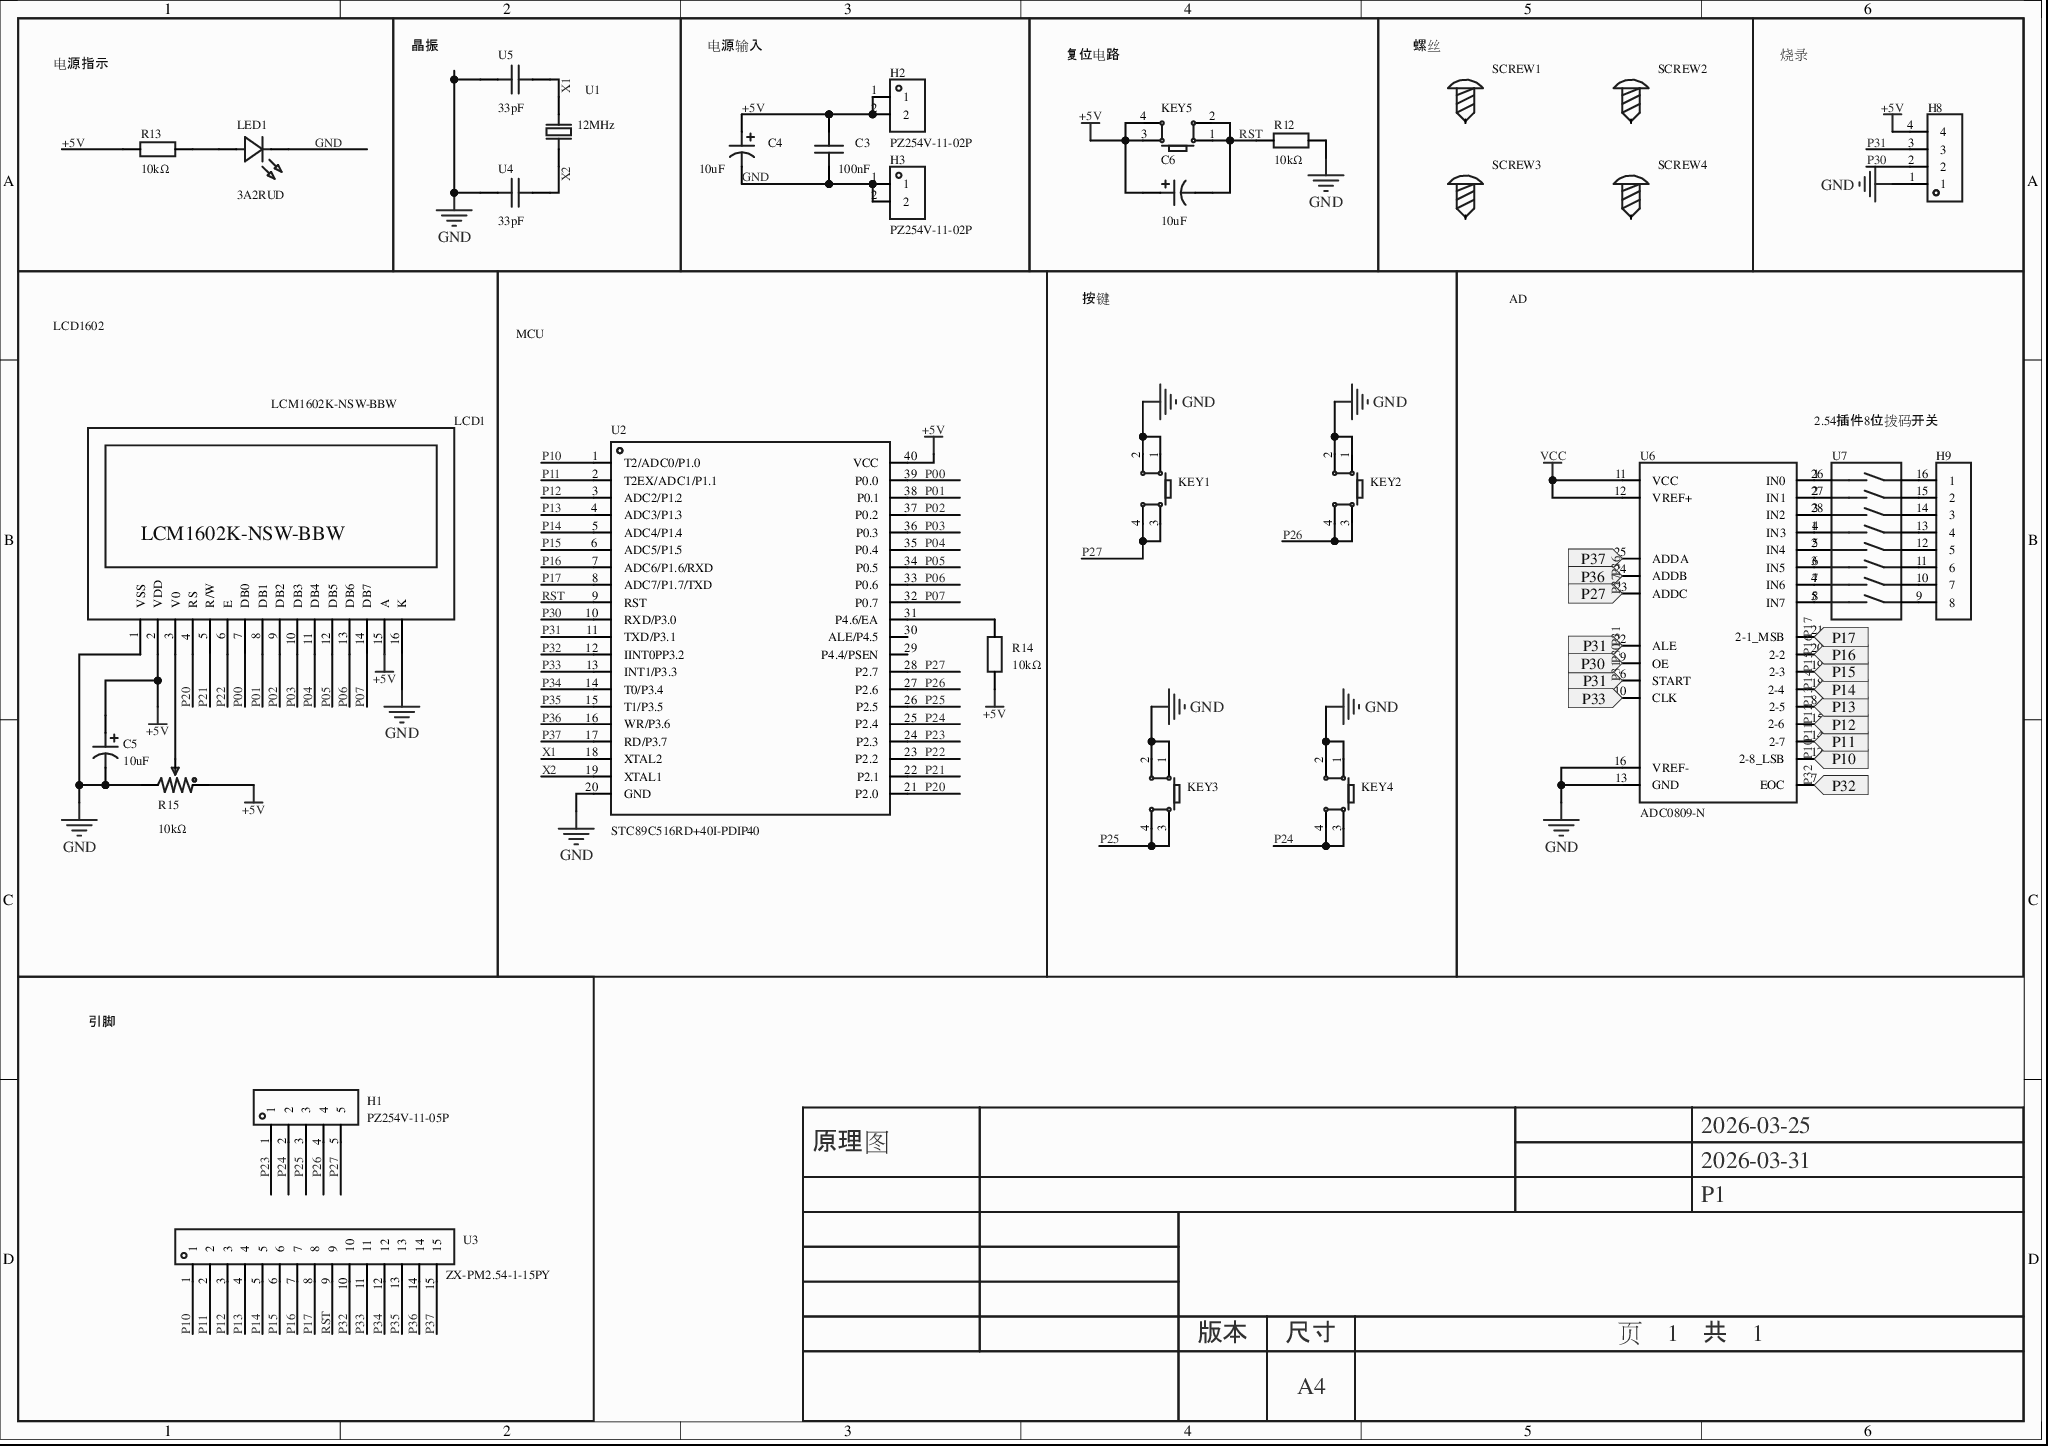
[diagram p0: MISC51962-3.schdoc]
# Altium project MISC51962-2.PrjPcb
1 sheet, 31 parts. Net scope: flat (ports and power ports of the same name join across sheets).
Board file: MISC51962.pcbdoc

## Sheet MISC51962-3.schdoc
size 297 x 209 mm; Version: V1.0; @Project Name: MISC51962; @Page Count: 1; @Update Date: 2026-04-15; @Create Date: 2026-04-15; @Schematic Name: MISC51962; @Page No: 1; @Board Name: MISC51962; @Create Time: 20:25:54; @Update Time: 20:28:01; Size: A4

### Parts
C3  100nF  [CAP-TH_L5.0-W2.5-P5.00-D1.0]
C4  10uF  [CAP-TH_BD5.0-P2.00-D0.5-FD-A]
C5  10uF  [CAP-TH_BD5.0-P2.00-D0.5-FD-A]
C6  10uF  [CAP-TH_BD5.0-P2.00-D0.5-FD-A]
H1  PZ254V-11-05P  [HDR-TH_5P-P2.54-V-M]
H2  PZ254V-11-02P  [HDR-TH_2P-P2.54-V-M]
H3  PZ254V-11-02P  [HDR-TH_2P-P2.54-V-M]
H8  (no value)  [HDR-TH_4P-P2.54-V-F]
H9  (no value)  [HDR-TH_8P-P2.54-V-F-1]
KEY1  (no value)  [SW-TH_4P-L6.0-W6.0-P4.50-LS6.5]
KEY2  (no value)  [SW-TH_4P-L6.0-W6.0-P4.50-LS6.5]
KEY3  (no value)  [SW-TH_4P-L6.0-W6.0-P4.50-LS6.5]
KEY4  (no value)  [SW-TH_4P-L6.0-W6.0-P4.50-LS6.5]
KEY5  (no value)  [SW-TH_4P-L6.0-W6.0-P4.50-LS6.5]
LCD1  LCM1602K-NSW-BBW  [MODULE-TH_LCM1602K]
LED1  3A2RUD  [LED-TH_BD3.5-P2.28_3A2RUC]
R12  10kΩ  [RES-TH_BD2.3-L6.5-P10.50-D0.5]
R13  10kΩ  [RES-TH_BD2.3-L6.5-P10.50-D0.5]
R14  10kΩ  [RES-TH_BD2.3-L6.5-P10.50-D0.5]
R15  10kΩ  [RES-ADJ-TH_3P-L10.0-W10.0-P2.50-L]
SCREW1  (no value)  [M3螺丝]
SCREW2  (no value)  [M3螺丝]
SCREW3  (no value)  [M3螺丝]
SCREW4  (no value)  [M3螺丝]
U1  12MHz  [HC-49S_L11.0-W4.7-P4.88]
U2  STC89C516RD+40I-PDIP40  [DIP-40_L52.3-W13.9-P2.54-LS15.2-BL]
U3  ZX-PM2.54-1-15PY  [HDR-TH_15P-P2.54-V-F]
U4  33pF  [CAP-TH_L5.0-W2.5-P5.08-D0.7]
U5  33pF  [CAP-TH_L5.0-W2.5-P5.08-D0.7]
U6  ADC0809-N  [PDIP-28_L36.0-W13.0-P2.54-LS15.5-BL]
U7  2.54插件8位拨码开关  [SW-TH_16P-L21.9-W9.9-P2.54-LS7.8]

### Blocks framed on the sheet
电源指示: LED1 R13
晶振: U1 U4 U5
电源输入: C3 C4 H2 H3
复位电路: C6 KEY5 R12
螺丝: SCREW1-SCREW4
烧录: H8
LCD1602: C5 LCD1 R15
MCU: R14 U2
按键: KEY1-KEY4
AD: H9 U6 U7
引脚: H1 U3

### Ports
P10 (in), P11 (in), P12 (in), P13 (in), P14 (in), P15 (in), P16 (in), P17 (in), P27 (in), P30 (in), P31 (in), P32 (in), P33 (in), P36 (in), P37 (in)

### Nets
+5V: C3.2 C4.1 C5.1 C6.1 H2.1 H2.2 H8.4 KEY5.3 KEY5.4 LCD1.2(VDD) LCD1.15(A) R13.2 R14.1 R15.1 U2.40(VCC)
GND: C3.1 C4.2 C5.2 H3.1 H3.2 H8.1 KEY1.1 KEY1.2 KEY2.1 KEY2.2 KEY3.1 KEY3.2 KEY4.1 KEY4.2 LCD1.1(VSS) LCD1.16(K) LED1.1(K) R12.1 R15.3 U2.20(GND) U4.1 U5.1 U6.13(GND) U6.16(VREF-)
VCC: U6.11(VCC) U6.12(VREF+)
P00: LCD1.7(DB0) U2.39(P0.0)
P01: LCD1.8(DB1) U2.38(P0.1)
P02: LCD1.9(DB2) U2.37(P0.2)
P03: LCD1.10(DB3) U2.36(P0.3)
P04: LCD1.11(DB4) U2.35(P0.4)
P05: LCD1.12(DB5) U2.34(P0.5)
P06: LCD1.13(DB6) U2.33(P0.6)
P07: LCD1.14(DB7) U2.32(P0.7)
P10: U2.1(T2/ADC0/P1.0) U3.1 U6.17(2-8_LSB) ; port P10
P11: U2.2(T2EX/ADC1/P1.1) U3.2 U6.14(2-7) ; port P11
P12: U2.3(ADC2/P1.2) U3.3 U6.15(2-6) ; port P12
P13: U2.4(ADC3/P1.3) U3.4 U6.8(2-5) ; port P13
P14: U2.5(ADC4/P1.4) U3.5 U6.18(2-4) ; port P14
P15: U2.6(ADC5/P1.5) U3.6 U6.19(2-3) ; port P15
P16: U2.7(ADC6/P1.6/RXD) U3.7 U6.20(2-2) ; port P16
P17: U2.8(ADC7/P1.7/TXD) U3.8 U6.21(2-1_MSB) ; port P17
P20: LCD1.4(RS) U2.21(P2.0)
P21: LCD1.5(R/W) U2.22(P2.1)
P22: LCD1.6(E) U2.23(P2.2)
P23: H1.1 U2.24(P2.3)
P24: H1.2 KEY4.3 KEY4.4 U2.25(P2.4)
P25: H1.3 KEY3.3 KEY3.4 U2.26(P2.5)
P26: H1.4 KEY2.3 KEY2.4 U2.27(P2.6)
P27: H1.5 KEY1.3 KEY1.4 U2.28(P2.7) U6.23(ADDC) ; port P27
P30: H8.2 U2.10(RXD/P3.0) U6.9(OE) ; port P30
P31: H8.3 U2.11(TXD/P3.1) U6.6(START) U6.22(ALE) ; port P31
P32: U2.12(IINT0PP3.2) U3.10 U6.7(EOC) ; port P32
P33: U2.13(INT1/P3.3) U3.11
P34: U2.14(T0/P3.4) U3.12
P35: U2.15(T1/P3.5) U3.13
P36: U2.16(WR/P3.6) U3.14 U6.24(ADDB) ; port P36
P37: U2.17(RD/P3.7) U3.15
RST: C6.2 KEY5.1 KEY5.2 R12.2 U2.9(RST) U3.9
X1: U1.2 U2.18(XTAL2) U5.2
X2: U1.1 U2.19(XTAL1) U4.2
NetH9_1: H9.1 U7.16
NetH9_2: H9.2 U7.15
NetH9_3: H9.3 U7.14
NetH9_4: H9.4 U7.13
NetH9_5: H9.5 U7.12
NetH9_6: H9.6 U7.11
NetH9_7: H9.7 U7.10
NetH9_8: H9.8 U7.9
NetLCD1_3: LCD1.3(V0) R15.2
NetLED1_2: LED1.2(A) R13.1
NetR14_2: R14.2 U2.31(P4.6/EA)
NetU6_1: U6.1(IN3) U7.4
NetU6_2: U6.2(IN4) U7.5
NetU6_3: U6.3(IN5) U7.6
NetU6_4: U6.4(IN6) U7.7
NetU6_5: U6.5(IN7) U7.8
NetU6_10: U6.10(CLK) ; port P33
NetU6_25: U6.25(ADDA) ; port P37
NetU6_26: U6.26(IN0) U7.1
NetU6_27: U6.27(IN1) U7.2
NetU6_28: U6.28(IN2) U7.3

Not connected (* = marked no-connect by the designer): SCREW1 1*; SCREW2 1*; SCREW3 1*; SCREW4 1*; U2 29(P4.4/PSEN)* 30(ALE/P4.5)*

### Notes on the sheet
- 2026-03-25
- 原理图
- 2026-03-31
- P1
- 版本
- 尺寸
- A4
- 页    1    共    1

### Library data of the parts
C3 = CC1H104MC1FD3F6C10MF: Manufacturer: Dersonic(德尔创); AddInBom: yes; Tolerance: ±20%; Voltage Rating: 50V; Pin Spacing: 5.08mm; Temperature Coefficient: Y5V; Body Thickness: 2.2mm; ModelId: 08e3d7481fc7486bb1b263873f51e1e1; ModelName: CAP-TH_BD5.0-W2.5-P5.08; ModelTransform: 224.652,98.425,0,0,0,0,-0.005,0,-137.795; Device: CC1H104MC1FD3F6C10MF; Symbol: CC1H104MC1FD3F6C10MF; FootprintName: CAP-TH_L5.0-W2.5-P5.00-D1.0; LCSC Part Name: 100nF ±20% 50V; SupplierPart: C254085; ManufacturerPart: CC1H104MC1FD3F6C10MF; Supplier Footprint: 插件,P=5.08mm; JLCPCB Part Class: 扩展库; Datasheet: https://item.szlcsc.com/datasheet/CC1H104MC1FD3F6C10MF/248635.html; Supplier: LCSC; ConvertToPcb: yes; Value: 100nF; Diameter: 6mm
C4-C6 = ERG50V10M5X11: Manufacturer: JIERR(捷而瑞); AddInBom: yes; Tolerance: ±20%; Voltage Rating: 50V; Ripple Current: 180mA@100kHz; Equivalent Series Resistance(ESR): 1.3Ω@100kHz; Pin Spacing: 2mm; Lifetime: 2000hrs@105℃; ModelId: fb608287dcd66704; ModelTransform: 0,0,0,0,0,0,0,0,0; Device: ERG50V10M5X11; Symbol: ERG50V10M5X11; FootprintName: CAP-TH_BD5.0-P2.00-D0.5-FD-A; LCSC Part Name: 10uF ±20% 50V; SupplierPart: C47344184; ManufacturerPart: ERG50V10M5X11; Supplier Footprint: 插件,D5xL11mm; JLCPCB Part Class: 扩展库; Datasheet: https://item.szlcsc.com/datasheet/ERG50V10M5X11/49556625.html; Supplier: LCSC; ConvertToPcb: yes; Value: 10uF; Diameter: 5mm; Height - Seated (Max): 11mm; Operating Temperature: -40℃~+105℃; ModelName: CAP-TH_BD5.0-P2.00-D0.5-FD-A
H1 = PZ254V-11-05P: Manufacturer: XFCN(兴飞); AddInBom: yes; Pin Structure: 1x5P; Pitch: 2.54mm; Circluar Pins/Square Pins: 方针; Current Rating: 3A; Voltage Rating (Max): 250V; ModelId: 47d466e4a34f4fc5bc626cf773a24dd5; ModelName: HDR-TH_5P-P2.54-M-LI-1X5P; ModelTransform: 499.999,100,0,0,0,0,0,0,-118.11; Device: PZ254V-11-05P; Symbol: PZ254V-11-05P; FootprintName: HDR-TH_5P-P2.54-V-M; LCSC Part Name: 1x5P 间距:2.54mm 方针 直插; SupplierPart: C492404; ManufacturerPart: PZ254V-11-05P; Supplier Footprint: 插件,P=2.54mm; JLCPCB Part Class: 扩展库; Datasheet: https://item.szlcsc.com/datasheet/PZ254V-11-05P/502960.html; Supplier: LCSC; ConvertToPcb: yes; Row Spacing: -; Mounting Type: 直插; Number of Rows: 单排; Number of Pins: 5P; Length of Mating Pin: 6mm; Insulation Height: 2.5mm; Length of End Connection Pin: 3mm; Contact Material: 黄铜; Contact Plating: -; Operating Temperature: -40℃~+105℃; Color: 黑色
H2 H3 = PZ254V-11-02P: Manufacturer: XFCN(兴飞); AddInBom: yes; Pin Structure: 1x2P; Pitch: 2.54mm; Circluar Pins/Square Pins: 方针; Current Rating: 3A; Voltage Rating (Max): 250V; ModelId: e35305ec3aa84b66b849f914b715e73f; ModelName: HDR2.54-M-LI-1X2P; ModelTransform: 200,100,0,0,0,0,0,0,-118.11; Device: PZ254V-11-02P; Symbol: PZ254V-11-02P; FootprintName: HDR-TH_2P-P2.54-V-M; LCSC Part Name: 1x2P 间距:2.54mm 方针 直插; SupplierPart: C492401; ManufacturerPart: PZ254V-11-02P; Supplier Footprint: 插件,P=2.54mm; JLCPCB Part Class: 扩展库; Datasheet: https://item.szlcsc.com/datasheet/PZ254V-11-02P/502957.html; Supplier: LCSC; ConvertToPcb: yes; Row Spacing: -; Mounting Type: 直插; Number of Rows: 单排; Number of Pins: 2P; Length of Mating Pin: 6mm; Insulation Height: 2.5mm; Length of End Connection Pin: 3mm; Contact Material: 黄铜; Contact Plating: -; Operating Temperature: -40℃~+105℃; Color: 黑色
H8 = HDR-F_2.54_1x4P: Symbol: 2.54-1*4P母; ConvertToPcb: yes; ModelId: 6a0dd8df310fbcc7; ModelTransform: 0,0,0,0,0,0,0,0,0; Device: HDR-F_2.54_1x4P; FootprintName: HDR-TH_4P-P2.54-V-F; AddInBom: yes; SupplierPart: C2718488; Supplier Footprint: 插件; ModelName: HDR-TH_4P-P2.54-V-F
H9 = HDR-F_2.54_1x8P: Symbol: Header-Female-2.54_1x8; AddInBom: yes; ModelId: 0f7e4d9227ef4fa08d5469c22cc70cdb; ModelName: HDR-F-2.54_1x8; ModelTransform: 799.99844,100,0,0,0,0,0,0,-118.11; Device: HDR-F_2.54_1x8P; ConvertToPcb: yes; FootprintName: HDR-TH_8P-P2.54-V-F-1; SupplierPart: C27438; Supplier Footprint: 插件
KEY1-KEY5 = Key_TH_6x6x6: Symbol: 轻触按键; ConvertToPcb: yes; ModelId: 20eee248bc684ccd8cbdbb1d0d91ec6f; ModelName: SW-TH_4P-L6.0-W6.0-H5.0-LS6.5-P4.50; ModelTransform: 236.22,323.03,0,90,0,0,0,0,-137.795; Device: Key_TH_6x6x6; FootprintName: SW-TH_4P-L6.0-W6.0-P4.50-LS6.5; AddInBom: yes; SupplierPart: C2837516; Supplier Footprint: 插件
LCD1 = LCM1602K-NSW-BBW: Manufacturer: LONTECH(厦门龙特); AddInBom: yes; Controller Type: KS0066U; Display Range: 64.5x16.4mm; Display Color: 蓝底白字; Voltage - Supply: 4.7V~5.5V；2.7V~5.3V; ModelId: 786352422ee40831; ModelTransform: 0,0,0,0,0,0,0,0,0; Device: LCM1602K-NSW-BBW; Symbol: LCM1602K-NSW-BBW; FootprintName: MODULE-TH_LCM1602K; LCSC Part Name: LCM1602K-NSW-BBW; SupplierPart: C83275; ManufacturerPart: LCM1602K-NSW-BBW; Supplier Footprint: -; JLCPCB Part Class: 扩展库; Datasheet: https://item.szlcsc.com/datasheet/LCM1602K-NSW-BBW/84439.html; Supplier: LCSC; ConvertToPcb: yes; Size: -; ModelName: MODULE-TH_LCM1602K
LED1 = 3A2RUD: Manufacturer: Guiguang light(桂光光电); AddInBom: yes; Lamp Holder Type: 3mm圆形灯头; Illumination Color: 红色; Voltage - Forward(Vf): 1.8V~2.2V; Forward Current: 20mA; Wavelength - Dominant: 620nm~625nm; Peak Wavelength: 625nm; Lens Color: 红色透镜; Luminous Intensity: 200mcd~400mcd; Viewing Angle: 30°; ModelId: 7dc1228e7ab44762a69569a9a69b2349; ModelTransform: 129.53171,137.754,0,0,0,0,-3.937,0,-196.85; Device: 3A2RUD; Symbol: 3A2RUD; FootprintName: LED-TH_BD3.5-P2.28_3A2RUC; LCSC Part Name: 3mm 红发红短脚; SupplierPart: C52034637; ManufacturerPart: 3A2RUD; Supplier Footprint: 插件,D=3mm; JLCPCB Part Class: 扩展库; Datasheet: https://item.szlcsc.com/datasheet/3A2RUD/54791005.html; Supplier: LCSC; ConvertToPcb: yes; Color Temperature: -; Operating Temperature: -40℃~+85℃; ModelName: LED-TH_BD3.5-P2.28_3A2RUC
R12-R14 = MF1/4W-10KΩ±1% T: Manufacturer: CCO(千志电子); Symbol: MF1/4W-10KΩ±1% T52; AddInBom: yes; Tolerance: ±1%; Voltage-Supply(Max): 250V; Power(Watts): 250mW; Temperature Coefficient: ±100ppm/℃; ModelId: 8e6c7ee8323443d1ab8f0504b6353c8c; ModelName: RES-TH_D2.3-L6.5-P10.50; ModelTransform: 431.1015,91.3384,0,0,0,0,0.197,0,-137.795; Device: MF1/4W-10KΩ±1% T; FootprintName: RES-TH_BD2.3-L6.5-P10.50-D0.5; LCSC Part Name: 10kΩ ±1% 250mW 金属膜电阻 圆柱状直插; SupplierPart: C119347; ManufacturerPart: MF1/4W-10KΩ±1% T; Supplier Footprint: 插件,D2.3xL6.5mm; JLCPCB Part Class: 扩展库; Datasheet: https://atta.szlcsc.com/upload/public/pdf/source/20190910/C427326_62A6D058BC0FF74963A2F22379CA06CE.pdf; Supplier: LCSC; ConvertToPcb: yes; Type: 金属膜电阻; Value: 10kΩ; Operating Temperature: -55℃~+155℃
R15 = 3296W-1-103: Manufacturer: BOCHEN(博晨); AddInBom: yes; Tolerance: ±10%; Power(Watts): 500mW; Temperature Coefficient: ±250ppm/℃; Number of Turns: 30; ModelId: b182808559bb43bda9e7de64b64134cb; ModelName: 3296W; ModelTransform: 374.015,188.976,0,180,0,0,0,0,-137.795; Device: 3296W-1-103; Symbol: 3296W-1-103; FootprintName: RES-ADJ-TH_3P-L10.0-W10.0-P2.50-L; LCSC Part Name: 10kΩ ±10%; SupplierPart: C118954; ManufacturerPart: 3296W-1-103; Supplier Footprint: 插件-3P,9.5x4.9mm; JLCPCB Part Class: 扩展库; Datasheet: https://item.szlcsc.com/datasheet/3296W-1-103/120223.html; Supplier: LCSC; ConvertToPcb: yes; Value: 10kΩ
SCREW1-SCREW4 = M3螺丝: ConvertToPcb: yes; SymbolName: 螺丝孔; Device: M3螺丝; AddInBom: yes; Supplier Footprint: 插件; FootprintName: M3螺丝
U1 = YG12MLBBE2X: Manufacturer: YJX(雅晶鑫); AddInBom: yes; Normal temperature Frequency Tolerance: ±10ppm; Load Capacitance: 20pF; Frequency Stability: ±30ppm; Equivalent Series Resistance(ESR): 40Ω; ModelId: 90d89857b3344bee9813507fec06adb2; ModelTransform: 435.0385,183.0705,0,0,0,0,0,0,-196.85; Device: YG12MLBBE2X; Symbol: YG12MLBBE2X; FootprintName: HC-49S_L11.0-W4.7-P4.88; LCSC Part Name: 49S 12M 20PF 10PPM; SupplierPart: C42441036; ManufacturerPart: YG12MLBBE2X; Supplier Footprint: HC-49S; Datasheet: https://atta.szlcsc.com/upload/public/pdf/source/20250109/7D5687D7E6E611B127181E4BD00ED56D.pdf; Supplier: LCSC; ConvertToPcb: yes; Type: 插件晶振; Value: 12MHz; Operating Temperature: -20℃~+70℃; ModelName: HC-49S_L11.0-W4.7-P4.88
U2 = STC89C516RD+40I-PDIP40: Manufacturer: STC; AddInBom: yes; CPU Core: 51系列; Program Storage Size: 61KB; Program Memory Type: FLASH; Number of I/O: 35; Voltage - Supply: 3.5V~5.5V; ModelId: 16d4686a009b4ddca948f91eddb57b14; ModelName: DIP-40_L52.3-W13.8-H4.0-LS15.24-P2.54; ModelTransform: 2059.051,615.743,0,0,0,0,0,0,-129.921; Device: STC89C516RD+40I-PDIP40; Symbol: STC89C516RD+40I-PDIP40; FootprintName: DIP-40_L52.3-W13.9-P2.54-LS15.2-BL; LCSC Part Name: STC89C516RD+40I-PDIP40; SupplierPart: C52225; ManufacturerPart: STC89C516RD+40I-PDIP40; Supplier Footprint: DIP-40; JLCPCB Part Class: 扩展库; Datasheet: https://atta.szlcsc.com/upload/public/pdf/source/20250219/C2F0DDDE7C5E9ADA5B33742D18630F09.pdf; Supplier: LCSC; ConvertToPcb: yes; Applications: -
U3 = ZX-PM2.54-1-15PY: Manufacturer: Megastar(兆星); AddInBom: yes; Holes Structure: 1x15P; Pitch: 2.54mm; Circular Hole / Square Hole: 方孔; Number of Positions: 15P; Current Rating: 3A; Holes Direction: 顶部; PIN Length: 3.2mm; ModelId: c5912b504ede9fc8; ModelTransform: 0,0,0,0,0,0,0,0,0; Device: ZX-PM2.54-1-15PY; Symbol: ZX-PM2.54-1-15PY; FootprintName: HDR-TH_15P-P2.54-V-F; LCSC Part Name: 1x15P 间距:2.54mm 直插; SupplierPart: C7499333; ManufacturerPart: ZX-PM2.54-1-15PY; Supplier Footprint: 插件,P=2.54mm; JLCPCB Part Class: 扩展库; Datasheet: https://item.szlcsc.com/datasheet/ZX-PM2.54-1-15PY/8573994.html; Supplier: LCSC; ConvertToPcb: yes; Row Spacing: -; Mounting Type: 直插; Number of Rows: 单排; Voltage Rating (Max): -; Insulation Height: 8.5mm; Contact Material: 黄铜; Contact Plating: 金; Operating Temperature: -40℃~+105℃; ModelName: HDR-TH_15P-P2.54-V-F
U4 U5 = CC1H330JC74DCH4B10MN: Manufacturer: Dersonic(德尔创); AddInBom: yes; Tolerance: ±5%; Voltage Rating: 50V; Pin Spacing: 5.08mm; Temperature Coefficient: NP0; Body Thickness: 2.2mm; ModelId: 3d005bb2736f4b028b929daf59d2a504; ModelName: CAP-TH_L5.0-W2.5-P5.08; ModelTransform: 222.8342,98.419,0,0,0,0,0,0,-118.11; Device: CC1H330JC74DCH4B10MN; Symbol: CC1H330JC74DCH4B10MN; FootprintName: CAP-TH_L5.0-W2.5-P5.08-D0.7; LCSC Part Name: 33pF ±5% 50V; SupplierPart: C254101; ManufacturerPart: CC1H330JC74DCH4B10MN; Supplier Footprint: 插件,P=5.08mm; JLCPCB Part Class: 扩展库; Datasheet: https://item.szlcsc.com/datasheet/CC1H330JC74DCH4B10MN/248651.html; Supplier: LCSC; ConvertToPcb: yes; Value: 33pF; Diameter: 4.7mm
U6 = ADC0809-N: AddInBom: yes; ModelId: 8c6e055233a1409a85cd0ee0657823a6; ModelTransform: 1417.32,617.91215,0,0,0,0,0,0,-133.858; Symbol: ADC0809-N; Device: ADC0809-N; LCSC Part Name: ADC0809-N; SupplierPart: C9900042594; ManufacturerPart: ADC0809-N; Supplier Footprint: R-PDIP-24; Supplier: LCSC; ConvertToPcb: yes; FootprintName: PDIP-28_L36.0-W13.0-P2.54-LS15.5-BL; ModelName: PDIP-28_L36.0-W13.0-P2.54-LS15.5-BL
U7 = 2.54插件8位拨码开关: AddInBom: yes; ModelId: 94e83a27dea64f9d9a0937b590be243d; ModelTransform: 862.203,387.7945,0,0,0,0,0,0,-157.48; Symbol: 2.54插件8位拨码开关; Device: 2.54插件8位拨码开关; LCSC Part Name: 2.54插件8位拨码开关; SupplierPart: C9900005795; ManufacturerPart: 2.54插件8位拨码开关; Supplier Footprint: 插件; JLCPCB Part Class: 扩展库; Supplier: LCSC; ConvertToPcb: yes; FootprintName: SW-TH_16P-L21.9-W9.9-P2.54-LS7.8; ModelName: SW-TH_16P-L21.9-W9.9-P2.54-LS7.8